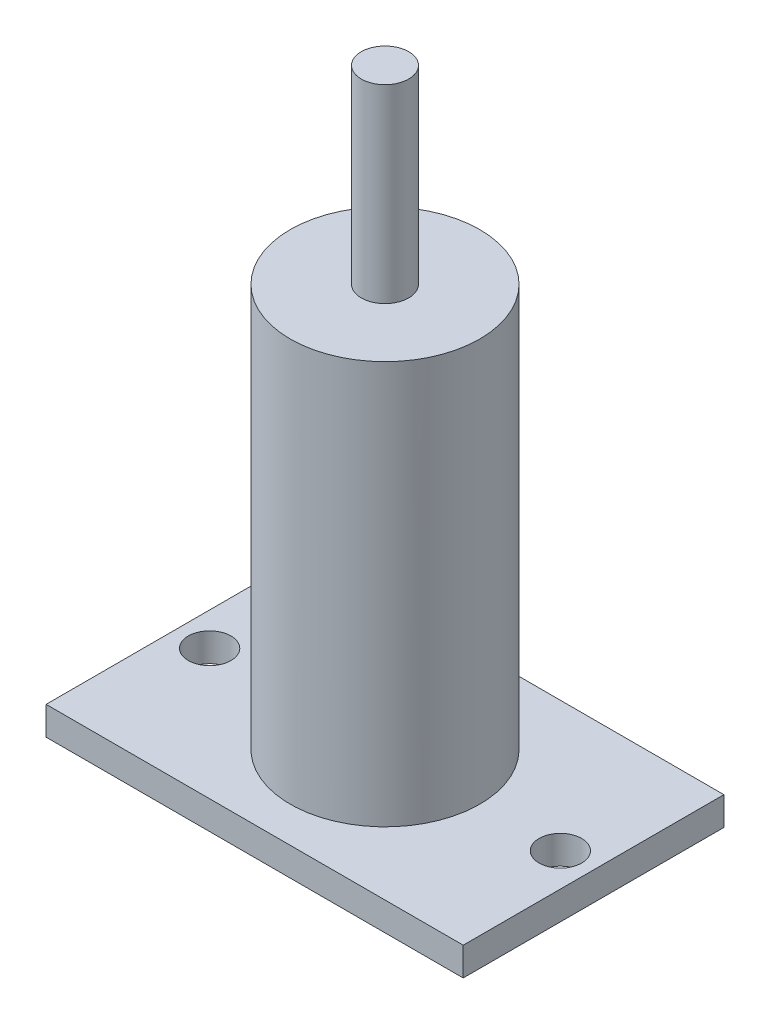
from build123d import *

# Parameters (mm, degrees)
SKETCH_1_W         = 88
SKETCH_1_H         = 55
EXTRUDE_1_DEPTH    = 6
HOLE_WIZARD_M8_1_D = 9
SKETCH_4_R         = 20
EXTRUDE_2_DEPTH    = 85
SKETCH_5_R         = 5
EXTRUDE_3_DEPTH    = 40


with BuildPart() as part:
    # 草图1 → 凸台-拉伸1 (new body)
    with BuildSketch(Plane(origin=(0, 0, 0), x_dir=(1, 0, 0), z_dir=(0, 1, 0))):
        Rectangle(SKETCH_1_W, SKETCH_1_H)
    extrude(amount=EXTRUDE_1_DEPTH)

    # M8 间隙孔1 (through all)
    with Locations(Plane(origin=(0, 6, 0), x_dir=(1, 0, 0), z_dir=(0, 1, 0))):
        with Locations((-37, 0), (37, 0)):
            Hole(HOLE_WIZARD_M8_1_D / 2)

    # 草图4 → 凸台-拉伸2 (add)
    with BuildSketch(Plane(origin=(0, 6, 0), x_dir=(1, 0, 0), z_dir=(0, 1, 0))):
        with Locations(Location((0, 0, 0), (0, 0, 90))):
            Circle(SKETCH_4_R)
    extrude(amount=EXTRUDE_2_DEPTH)

    # 草图5 → 凸台-拉伸3 (add)
    with BuildSketch(Plane(origin=(0, 91, 0), x_dir=(1, 0, 0), z_dir=(0, 1, 0))):
        with Locations(Location((0, 0, 0), (0, 0, 270))):
            Circle(SKETCH_5_R)
    extrude(amount=EXTRUDE_3_DEPTH)


solid = part.part
